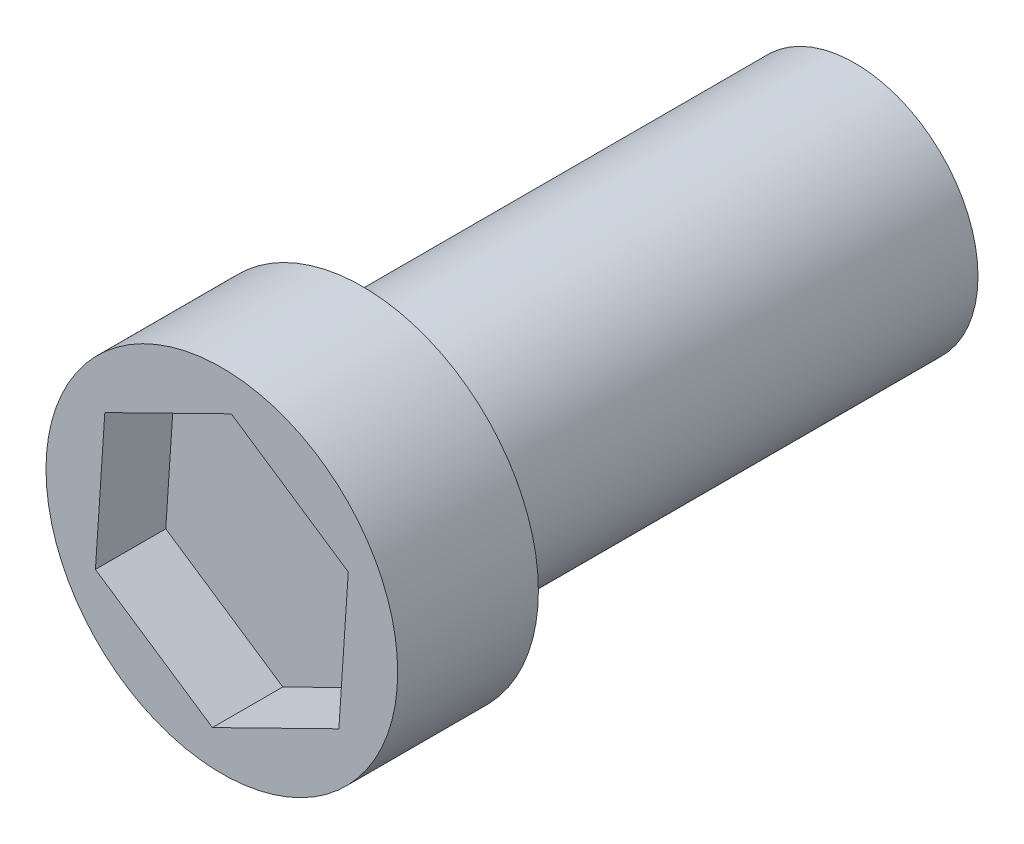
SolidWorks part; units mm, degrees
ref_plane "Front Plane" through (0, 0, 0) normal (0, 0, 1) x (1, 0, 0)
ref_plane "Top Plane" through (0, 0, 0) normal (0, 1, 0) x (1, 0, 0)
ref_plane "Right Plane" through (0, 0, 0) normal (1, 0, 0) x (0, 0, -1)
sketch "Sketch1" plane through (0, 0, 0) normal (0, 0, 1) x (1, 0, 0)
  circle A0 centre (0, 0) radius 2.5
  dimension "D1" = 5
extrude "Boss-Extrude1" add sketch "Sketch1" along normal blind 2
sketch "Sketch2" plane through (0, 0, 2) normal (0, 0, 1) x (1, 0, 0)
  line L1 (1.6637, -1.115) -> (1.7974, 0.8833)
  line L2 (1.7974, 0.8833) -> (0.1337, 1.9983)
  line L3 (0.1337, 1.9983) -> (-1.6637, 1.115)
  line L4 (-1.6637, 1.115) -> (-1.7974, -0.8833)
  line L5 (-1.7974, -0.8833) -> (-0.1337, -1.9983)
  line L6 (-0.1337, -1.9983) -> (1.6637, -1.115)
  circle A0 centre (0, 0) radius 1.7344 construction
extrude "Cut-Extrude1" cut sketch "Sketch2" against normal blind 1
sketch "Sketch3" plane through (0, 0, 0) normal (0, 0, -1) x (-1, 0, 0)
  circle A0 centre (0, 0) radius 1.75
  dimension "D1" = 3.5
extrude "Boss-Extrude2" add sketch "Sketch3" along normal blind 7
